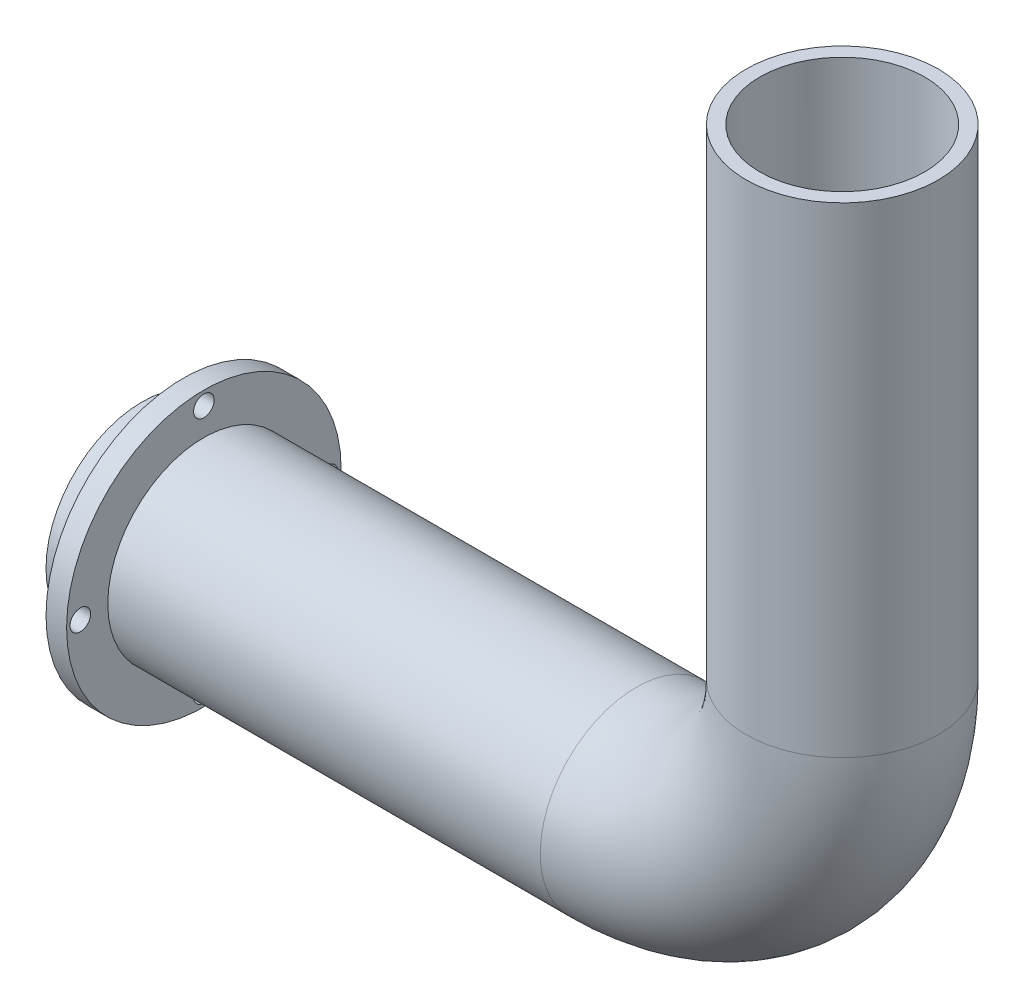
from build123d import *

# Parameters (mm, degrees)
SWEEP1_PROFILE_R    = 14
SHELL1_T            = -2
BOSS_EXTRUDE1_START = -6
SKETCH6_R           = 20
SKETCH6_R_2         = 12
SKETCH6_R_3         = 1.5
BOSS_EXTRUDE1_DEPTH = 3


with BuildPart() as part:
    # Sweep1: sweep along a path in Sketch1
    with BuildLine(Plane.XY) as sweep1_path:
        Line((0, 0), (0, -70))
        ThreePointArc((0, -70), (-8.786796564, -91.213203436), (-30, -100))
        Line((-30, -100), (-102, -100))
    # Sweep1 profile (on start of the path) → Sweep1 (sweep)
    with BuildSketch(Plane(origin=(0, 0, 0), x_dir=(-1, 0, 0), z_dir=(0, -1, 0))):
        Circle(SWEEP1_PROFILE_R)
    sweep(path=sweep1_path.line)

    # Shell1
    shell1_openings = [part.faces().sort_by_distance(p)[0] for p in [
        (-102, -100, 0),
        (0, 0, 0),
    ]]
    offset(amount=SHELL1_T, openings=shell1_openings, kind=Kind.INTERSECTION)

    # Sketch6 → Boss-Extrude1 (add)
    with BuildSketch(Plane.ZY.offset(102).offset(BOSS_EXTRUDE1_START)):
        with Locations((0, -100)):
            Circle(SKETCH6_R)
        with Locations(Location((0, -100, 0), (0, 0, 270))):
            Circle(SKETCH6_R_2, mode=Mode.SUBTRACT)
        with Locations((0, -82)):
            Circle(SKETCH6_R_3, mode=Mode.SUBTRACT)
        with Locations((18, -100)):
            Circle(SKETCH6_R_3, mode=Mode.SUBTRACT)
        with Locations((0, -118)):
            Circle(SKETCH6_R_3, mode=Mode.SUBTRACT)
        with Locations((-18, -100)):
            Circle(SKETCH6_R_3, mode=Mode.SUBTRACT)
    extrude(amount=-BOSS_EXTRUDE1_DEPTH)


solid = part.part
